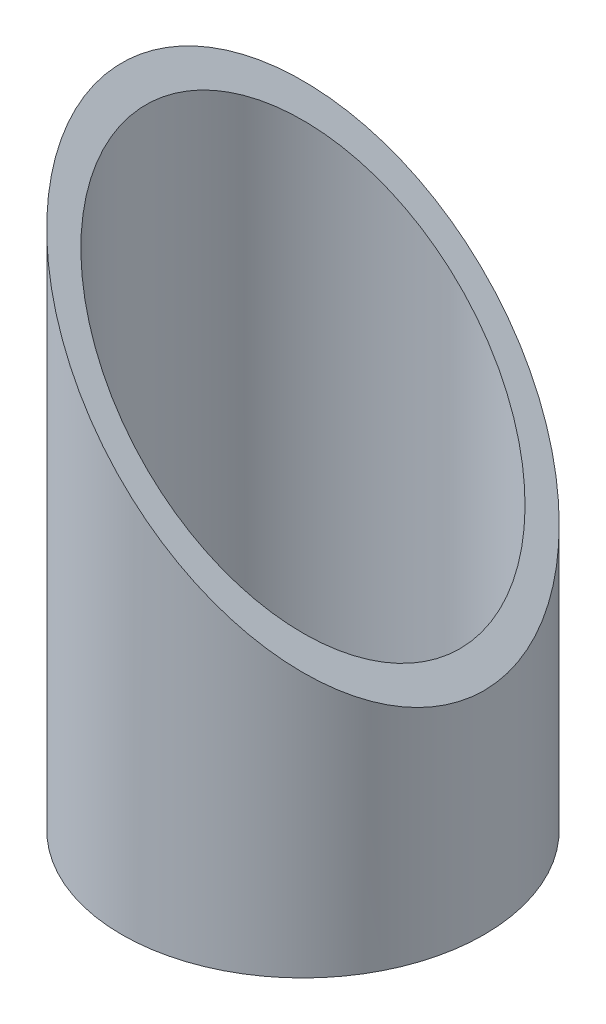
from build123d import *

# Parameters (mm, degrees)
SKETCH1_R               = 30
SKETCH1_R_2             = 26
BOSS_EXTRUDE1_DEPTH     = 95
CUT_EXTRUDE1_DEPTH      = 105.043260233
CUT_EXTRUDE1_DEPTH_BACK = 105.043260233


with BuildPart() as part:
    # Sketch1 → Boss-Extrude1 (new body)
    with BuildSketch(Plane(origin=(0, 0, 0), x_dir=(1, 0, 0), z_dir=(0, 1, 0))):
        with Locations(Location((0, 0, 0), (0, 0, 270))):
            Circle(SKETCH1_R)
        with Locations(Location((0, 0, 0), (0, 0, 270))):
            Circle(SKETCH1_R_2, mode=Mode.SUBTRACT)
    extrude(amount=BOSS_EXTRUDE1_DEPTH)

    # Sketch2 → Cut-Extrude1 (cut, two sides: drawn at the far end of the back side and taken through both)
    with BuildSketch(Plane.XY.offset(-CUT_EXTRUDE1_DEPTH_BACK)):
        Polygon((-195.973553633, 260.973553633), (-30, 95), (45.712319076, 19.287680924), (211.685872708, -146.685872708), (543.632979974, 185.261234557), (135.973553633, 592.920660898), align=None)
    extrude(amount=CUT_EXTRUDE1_DEPTH + CUT_EXTRUDE1_DEPTH_BACK, mode=Mode.SUBTRACT)


solid = part.part
